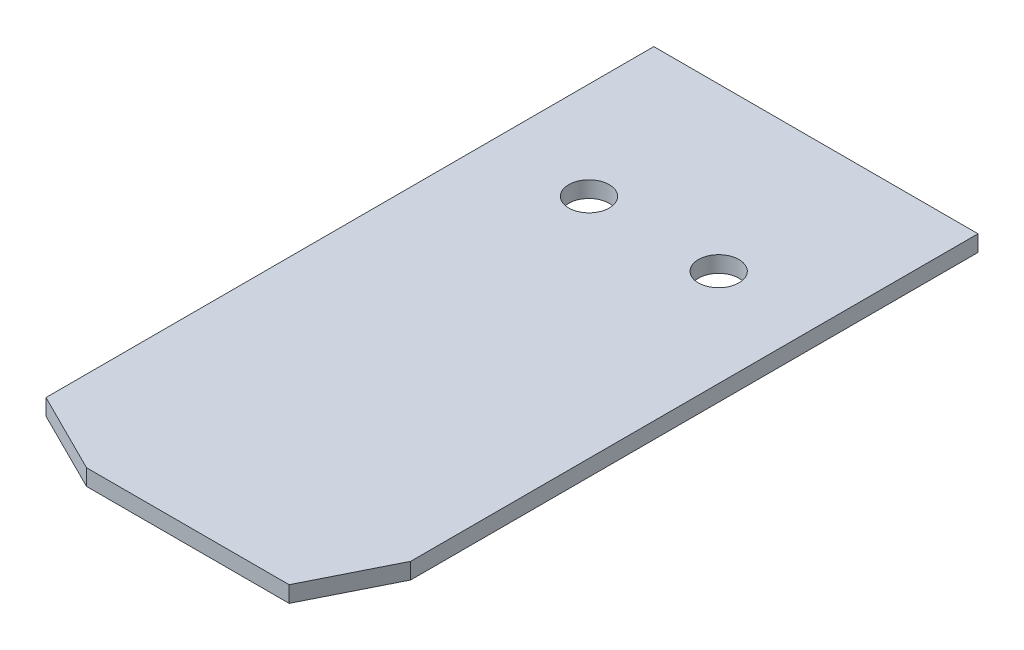
SolidWorks part; units mm, degrees
ref_plane "Front Plane" through (0, 0, 0) normal (0, 0, 1) x (1, 0, 0)
ref_plane "Top Plane" through (0, 0, 0) normal (0, 1, 0) x (1, 0, 0)
ref_plane "Right Plane" through (0, 0, 0) normal (1, 0, 0) x (0, 0, -1)
sketch "Sketch1" plane through (0, 0, 0) normal (0, 1, 0) x (1, 0, 0)
  line L1 (-20, 40) -> (20, 40)
  line L2 (-20, 40) -> (-20, -40)
  line L3 (-20, -40) -> (20, -40)
  line L4 (20, 40) -> (20, -40)
  line L5 (-20, 40) -> (20, -40) construction
  line L6 (-20, -40) -> (20, 40) construction
  point P0 (0, 0)
  dimension "D1" = 40
  dimension "D2" = 80
extrude "Boss-Extrude1" add sketch "Sketch1" along normal blind 2
sketch "Sketch2" plane through (0, 0, 0) normal (0, -1, 0) x (1, 0, 0)
  circle A0 centre (8, -20) radius 2.5
  circle A1 centre (-8, -20) radius 2.5
  dimension "D1" = 5
extrude "Cut-Extrude1" cut sketch "Sketch2" against normal blind 10
chamfer "Chamfer1" distance 5 distance2 10 2 edges at (20, 1, 40) (-20, 1, 40)
